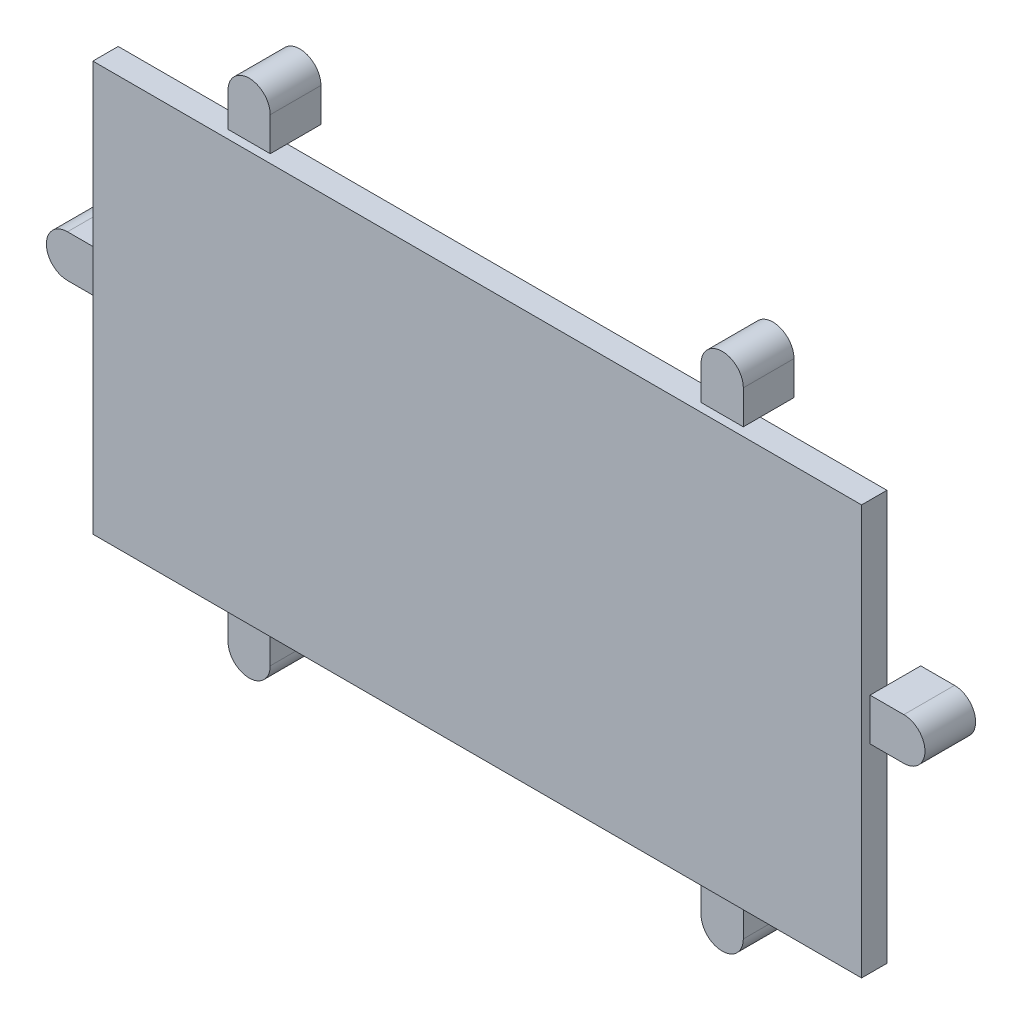
from build123d import *

# Parameters (mm, degrees)
SKETCH1_W           = 182
SKETCH1_H           = 97
BOSS_EXTRUDE1_DEPTH = 6
BOSS_EXTRUDE2_DEPTH = 12


with BuildPart() as part:
    # Sketch1 → Boss-Extrude1 (new body)
    with BuildSketch(Plane.XY):
        with Locations((47.006685832, -9.482901158)):
            Rectangle(SKETCH1_W, SKETCH1_H)
    extrude(amount=BOSS_EXTRUDE1_DEPTH)

    # Sketch2 → Boss-Extrude2 (add)
    with BuildSketch(Plane.XY.offset(-8)):
        with BuildLine():
            Line((108.006685832, -65.982901158), (108.006685832, -57.982901158))
            Line((108.006685832, -57.982901158), (98.006685832, -57.982901158))
            Line((98.006685832, -57.982901158), (98.006685832, -65.982901158))
            ThreePointArc((98.006685832, -65.982901158), (103.006685832, -70.982901158), (108.006685832, -65.982901158))
        make_face()
        with BuildLine():
            Line((138.006685832, -0.982901158), (138.006685832, -10.982901158))
            Line((138.006685832, -10.982901158), (146.006685832, -10.982901158))
            ThreePointArc((146.006685832, -10.982901158), (151.006685832, -5.982901158), (146.006685832, -0.982901158))
            Line((146.006685832, -0.982901158), (138.006685832, -0.982901158))
        make_face()
        with BuildLine():
            Line((108.006685832, 39.017098842), (108.006685832, 47.017098842))
            ThreePointArc((108.006685832, 47.017098842), (103.006685832, 52.017098842), (98.006685832, 47.017098842))
            Line((98.006685832, 47.017098842), (98.006685832, 39.017098842))
            Line((98.006685832, 39.017098842), (108.006685832, 39.017098842))
        make_face()
        with BuildLine():
            Line((-13.993314168, 47.017098842), (-13.993314168, 39.017098842))
            Line((-13.993314168, 39.017098842), (-3.993314168, 39.017098842))
            Line((-3.993314168, 39.017098842), (-3.993314168, 47.017098842))
            ThreePointArc((-3.993314168, 47.017098842), (-8.993314168, 52.017098842), (-13.993314168, 47.017098842))
        make_face()
        with BuildLine():
            Line((-43.993314168, -10.982901158), (-43.993314168, -0.982901158))
            Line((-43.993314168, -0.982901158), (-51.993314168, -0.982901158))
            ThreePointArc((-51.993314168, -0.982901158), (-56.993314168, -5.982901158), (-51.993314168, -10.982901158))
            Line((-51.993314168, -10.982901158), (-43.993314168, -10.982901158))
        make_face()
        with BuildLine():
            Line((-13.993314168, -57.982901158), (-13.993314168, -65.982901158))
            ThreePointArc((-13.993314168, -65.982901158), (-8.993314168, -70.982901158), (-3.993314168, -65.982901158))
            Line((-3.993314168, -65.982901158), (-3.993314168, -57.982901158))
            Line((-3.993314168, -57.982901158), (-13.993314168, -57.982901158))
        make_face()
    extrude(amount=BOSS_EXTRUDE2_DEPTH)


solid = part.part
